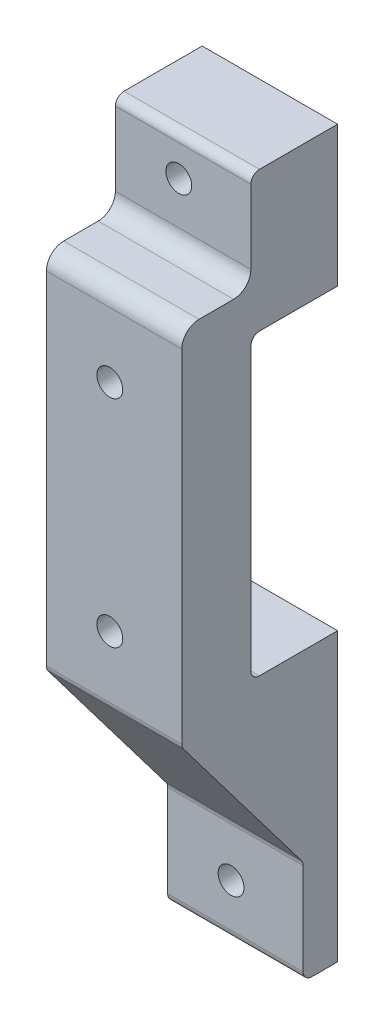
SolidWorks part; units mm, degrees
ref_plane "Front Plane" through (0, 0, 0) normal (0, 0, 1) x (1, 0, 0)
ref_plane "Top Plane" through (0, 0, 0) normal (0, 1, 0) x (1, 0, 0)
ref_plane "Right Plane" through (0, 0, 0) normal (1, 0, 0) x (0, 0, -1)
other "Configuration Table"
sketch "Sketch1" plane through (0, 0, 0) normal (0, 0, 1) x (1, 0, 0)
  line L1 (-8.35, 20) -> (8.35, 20)
  line L2 (-8.35, 20) -> (-8.35, -20)
  line L3 (-8.35, -20) -> (8.35, -20)
  line L4 (8.35, 20) -> (8.35, -20)
  line L5 (0, -20) -> (0, 20) construction
  line L6 (-8.35, 0) -> (8.35, 0) construction
  point P0 (0, 0)
  dimension "D1" = 16.7
  dimension "D2" = 40
extrude "Boss-Extrude1" add sketch "Sketch1" along normal blind 2
sketch "Sketch12" plane through (0, 0, 0) normal (0, 0, -1) x (-1, 0, 0)
  line L4 (-8.35, -20) -> (8.35, -20)
  line L5 (8.35, -20) -> (8.35, 20)
  line L6 (-8.35, -20) -> (8.35, -20)
  line L7 (-8.35, 20) -> (-8.35, -20)
  line L9 (8.35, -20) -> (8.35, 20)
  line L11 (-8.35, 20) -> (-8.35, -20)
  line L12 (8.35, 20) -> (-8.35, 20)
  line L13 (8.35, 20) -> (-8.35, 20)
  dimension "D1" = 0
extrude "Boss-Extrude4" add sketch "Sketch12" along normal blind 6
sketch "Sketch15" plane through (0, 0, 2) normal (0, 0, 1) x (1, 0, 0)
  line L0 (0, 20) -> (0, -20) construction
  line L1 (8.35, 20) -> (-8.35, 20) construction
  line L2 (-8.35, -20) -> (8.35, -20) construction
  circle A0 centre (0, 12.5) radius 1.5
  circle A1 centre (0, -12.5) radius 1.5
  dimension "D1" = 3
  dimension "D3" = 3
  dimension "D2" = 25
  dimension "D4" = 7.5
extrude "Cut-Extrude3" cut sketch "Sketch15" against normal through all
sketch "Sketch16" plane through (0, 0, -6) normal (0, 0, -1) x (-1, 0, 0)
  line L0 (-8.35, 20) -> (-8.35, -20) construction
  line L1 (-8.35, 17.3013) -> (8.35, 17.3013)
  line L2 (-8.35, 17.3013) -> (-8.35, 30.5519)
  line L3 (-8.35, 30.5519) -> (8.35, 30.5519)
  line L4 (8.35, 17.3013) -> (8.35, 30.5519)
  line L5 (8.35, -20) -> (8.35, 20) construction
  line L6 (8.35, 0) -> (-8.35, 0) construction
  line L7 (8.35, -17.3013) -> (8.35, -30.5519)
  line L8 (-8.35, -30.5519) -> (8.35, -30.5519)
  line L9 (-8.35, -17.3013) -> (-8.35, -30.5519)
  line L10 (-8.35, -17.3013) -> (8.35, -17.3013)
extrude "Boss-Extrude5" add sketch "Sketch16" along normal blind 6
sketch "Sketch21" plane through (0, 0, -12) normal (0, 0, -1) x (-1, 0, 0)
  line L0 (8.35, -17.3013) -> (-8.35, -17.3013) construction
  line L1 (-8.35, -17.3013) -> (-8.35, -30.5519) construction
  line L2 (-8.35, -30.5519) -> (8.35, -30.5519) construction
  line L3 (8.35, -30.5519) -> (8.35, -17.3013) construction
  line L4 (-8.35, 30.5519) -> (-8.35, 17.3013) construction
  line L5 (-8.35, 17.3013) -> (8.35, 17.3013) construction
  line L6 (8.35, 17.3013) -> (8.35, 30.5519) construction
  line L7 (8.35, 30.5519) -> (-8.35, 30.5519) construction
  line L8 (8.35, -17.3013) -> (-8.35, -17.3013)
  line L9 (-8.35, -17.3013) -> (-8.35, -30.5519)
  line L10 (-8.35, -30.5519) -> (8.35, -30.5519)
  line L11 (8.35, -30.5519) -> (8.35, -17.3013)
  line L12 (-8.35, 30.5519) -> (-8.35, 17.3013)
  line L13 (-8.35, 17.3013) -> (8.35, 17.3013)
  line L14 (8.35, 17.3013) -> (8.35, 30.5519)
  line L15 (8.35, 30.5519) -> (-8.35, 30.5519)
extrude "Boss-Extrude10" add sketch "Sketch21" along normal blind 4.06
sketch "Sketch22" plane through (0, -30.5519, 0) normal (0, -1, 0) x (1, 0, 0)
  line L0 (8.35, -16.06) -> (8.35, -6) construction
  line L1 (-8.35, -16.06) -> (8.35, -16.06)
  line L2 (-8.35, -16.06) -> (-8.35, -12.06)
  line L3 (-8.35, -12.06) -> (8.35, -12.06)
  line L4 (8.35, -16.06) -> (8.35, -12.06)
  dimension "D1" = 4
extrude "Boss-Extrude11" add sketch "Sketch22" along normal blind 20
sketch "Sketch23" plane through (8.35, 0, 0) normal (1, 0, 0) x (0, 0, -1)
  line L0 (-2, -20) -> (6, -30.5519)
  line L1 (6, -30.5519) -> (12.06, -38.545)
  line L2 (12.06, -50.5519) -> (12.06, -30.5519) construction
  line L3 (12.06, -38.545) -> (12.06, -20)
  line L4 (12.06, -20) -> (-2, -20)
  line L5 (-19.4535, 0) -> (26.9032, 0) construction
extrude "Boss-Extrude12" add sketch "Sketch23" along direction (1, 0, 0) on the side against the normal up to surface (16.7 mm away)
sketch "Sketch24" plane through (0, 0, -12.06) normal (0, 0, 1) x (1, 0, 0)
  line L0 (-24.769, 0) -> (48.6587, 0) construction
  line L1 (-8.35, -44.5485) -> (8.35, -44.5485) construction
  line L2 (-8.35, -50.5519) -> (-8.35, -38.545) construction
  line L3 (8.35, -50.5519) -> (8.35, -38.545) construction
  line L4 (-8.35, 44.5485) -> (8.35, 44.5485) construction
  circle A0 centre (0, -44.5485) radius 1.5
  circle A1 centre (0, 44.5485) radius 1.5
  point P11 (0, -44.5485)
  dimension "D1" = 3
extrude "Cut-Extrude5" cut sketch "Sketch24" against normal through all
sketch "Sketch25" plane through (0, 20, 0) normal (0, 1, 0) x (1, 0, 0)
  line L4 (8.35, -2) -> (8.35, 6)
  line L5 (8.35, 6) -> (-8.35, 6)
  line L6 (-8.35, 6) -> (-8.35, -2)
  line L7 (-8.35, -2) -> (8.35, -2)
  line L8 (8.35, -2) -> (8.35, 6)
  line L9 (8.35, 6) -> (-8.35, 6)
  line L10 (-8.35, 6) -> (-8.35, -2)
  line L11 (-8.35, -2) -> (8.35, -2)
  dimension "D1" = 0
extrude "Boss-Extrude13" add sketch "Sketch25" along normal blind 2
fillet "Fillet1" radius 2 1 edges at (0, 22, 2)
fillet "Fillet2" radius 2 1 edges at (0, 22, -6)
sketch "Sketch27" plane through (0, 30.5519, 0) normal (0, 1, 0) x (1, 0, 0)
  line L4 (-8.35, 6) -> (8.35, 6)
  line L5 (8.35, 6) -> (8.35, 16.06)
  line L6 (8.35, 16.06) -> (-8.35, 16.06)
  line L7 (-8.35, 16.06) -> (-8.35, 6)
  line L8 (-8.35, 6) -> (8.35, 6)
  line L9 (8.35, 6) -> (8.35, 16.06)
  line L10 (8.35, 16.06) -> (-8.35, 16.06)
  line L11 (-8.35, 16.06) -> (-8.35, 6)
  dimension "D1" = 0
extrude "Boss-Extrude14" add sketch "Sketch27" along normal blind 3
sketch "Sketch26" plane through (0, 0, -6) normal (0, 0, 1) x (1, 0, 0)
  line L0 (8.35, 33.5519) -> (8.35, 24) construction
  circle A0 centre (0, 28.9515) radius 1.5
  circle A1 centre (0, -44.5485) radius 1.5 construction
  circle A2 centre (0, -44.5485) radius 1.5 construction
  dimension "D1" = 3
  dimension "D2" = 73.5
  dimension "D3" = 8.35
extrude "Cut-Extrude6" cut sketch "Sketch26" against normal through all
sketch "Sketch28" plane through (-8.35, 0, 0) normal (-1, 0, 0) x (0, 0, 1)
  line L12 (2, -20) -> (2, 20)
  line L13 (0, 22) -> (-4, 22)
  line L14 (-6, 24) -> (-6, 33.5519)
  line L15 (-6, 33.5519) -> (-16.06, 33.5519)
  line L16 (-16.06, 33.5519) -> (-16.06, 17.3013)
  line L17 (-16.06, 17.3013) -> (-6, 17.3013)
  line L18 (-6, 17.3013) -> (-6, -17.3013)
  line L19 (-6, -17.3013) -> (-16.06, -17.3013)
  line L20 (-16.06, -17.3013) -> (-16.06, -50.5519)
  line L21 (-16.06, -50.5519) -> (-12.06, -50.5519)
  line L22 (-12.06, -50.5519) -> (-12.06, -38.545)
  line L23 (-12.06, -38.545) -> (2, -20)
  line L24 (2, -20) -> (2, 20)
  line L25 (0, 22) -> (-4, 22)
  line L26 (-6, 24) -> (-6, 33.5519)
  line L27 (-6, 33.5519) -> (-16.06, 33.5519)
  line L28 (-16.06, 33.5519) -> (-16.06, 17.3013)
  line L29 (-16.06, 17.3013) -> (-6, 17.3013)
  line L30 (-6, 17.3013) -> (-6, -17.3013)
  line L31 (-6, -17.3013) -> (-16.06, -17.3013)
  line L32 (-16.06, -17.3013) -> (-16.06, -50.5519)
  line L33 (-16.06, -50.5519) -> (-12.06, -50.5519)
  line L34 (-12.06, -50.5519) -> (-12.06, -38.545)
  line L35 (-12.06, -38.545) -> (2, -20)
  arc A2 (2, 20) -> (0, 22) centre (0, 20) ccw
  arc A3 (-6, 24) -> (-4, 22) centre (-4, 24) ccw
  arc A4 (2, 20) -> (0, 22) centre (0, 20) ccw
  arc A5 (-6, 24) -> (-4, 22) centre (-4, 24) ccw
  dimension "D1" = 0
extrude "Cut-Extrude7" cut sketch "Sketch28" against normal blind 1
fillet "Fillet3" radius 1 6 edges at (0.5, -17.3013, -6) (0.5, 17.3013, -6) (0.5, -50.5519, -12.06) (0.5, 33.5519, -6) (0.5, -38.545, -12.06) (0.5, -20, 2)
